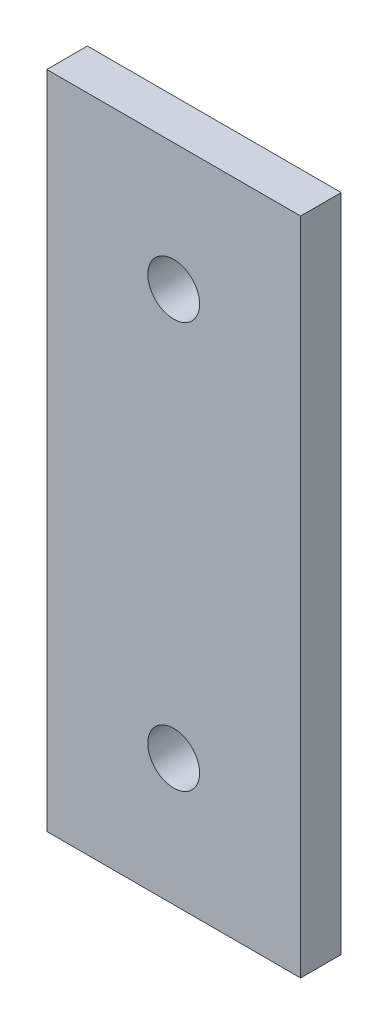
from build123d import *

# Parameters (mm, degrees)
SKETCH1_W              = 50
SKETCH1_H              = 130
BOSS_EXTRUDE1_DEPTH    = 8
M12_TAPPED_HOLE1_D     = 10.2
M12_TAPPED_HOLE1_DEPTH = 29.25
M12_TAPPED_HOLE1_TIP   = 3.064389157


with BuildPart() as part:
    # Sketch1 → Boss-Extrude1 (new body)
    with BuildSketch(Plane.XY):
        Rectangle(SKETCH1_W, SKETCH1_H)
    extrude(amount=BOSS_EXTRUDE1_DEPTH)

    # M12 Tapped Hole1
    with Locations(Plane.XY.offset(8)):
        with Locations((0, 40), (0, -40)):
            Hole(M12_TAPPED_HOLE1_D / 2, depth=M12_TAPPED_HOLE1_DEPTH)
            with Locations((0, 0, -(M12_TAPPED_HOLE1_DEPTH + M12_TAPPED_HOLE1_TIP / 2))):  # 118° drill point
                Cone(0, M12_TAPPED_HOLE1_D / 2, M12_TAPPED_HOLE1_TIP, mode=Mode.SUBTRACT)


solid = part.part
